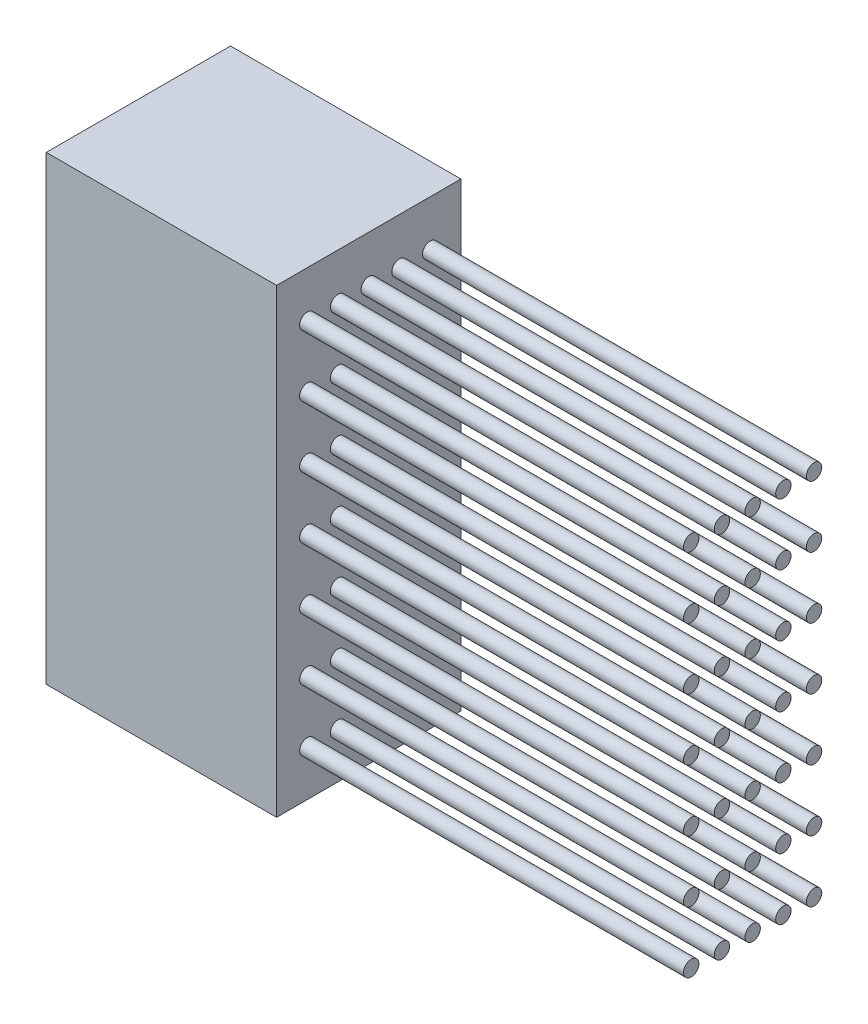
SolidWorks part; units mm, degrees
ref_plane "前视基准面" through (0, 0, 0) normal (0, 0, 1) x (1, 0, 0)
ref_plane "上视基准面" through (0, 0, 0) normal (0, 1, 0) x (1, 0, 0)
ref_plane "右视基准面" through (0, 0, 0) normal (1, 0, 0) x (0, 0, -1)
sketch "草图1" plane through (0, 0, 0) normal (0, 0, 1) x (1, 0, 0)
  line L1 (-7.5, -15) -> (7.5, -15)
  line L2 (-7.5, -15) -> (-7.5, 15)
  line L3 (-7.5, 15) -> (7.5, 15)
  line L4 (7.5, -15) -> (7.5, 15)
  line L5 (-7.5, -15) -> (7.5, 15) construction
  line L6 (-7.5, 15) -> (7.5, -15) construction
  point P0 (0, 0)
  dimension "D1" = 15
  dimension "D2" = 30
extrude "凸台-拉伸1" add sketch "草图1" along normal mid plane 12
sketch "草图2" plane through (7.5, 0, 0) normal (1, 0, 0) x (0, 0, -1)
  line L0 (0, 0) -> (0, 15) construction
  line L1 (-6, 15) -> (6, 15) construction
  circle A2 centre (-4, 0) radius 0.5
  circle A3 centre (-2, 0) radius 0.5
  circle A4 centre (0, 0) radius 0.5
  circle A5 centre (2, 0) radius 0.5
  circle A6 centre (4, 0) radius 0.5
  dimension "D1" = 1
  dimension "D2" = 2
  dimension "D3" = 2
extrude "凸台-拉伸2" add sketch "草图2" along normal blind 25
pattern_linear "阵列(线性)1" count 4 spacing 4 along (0, -1, 0) of "凸台-拉伸2"
mirror "镜向1" about plane through (0, 0, 0) normal (0, 1, 0) of "阵列(线性)1"
